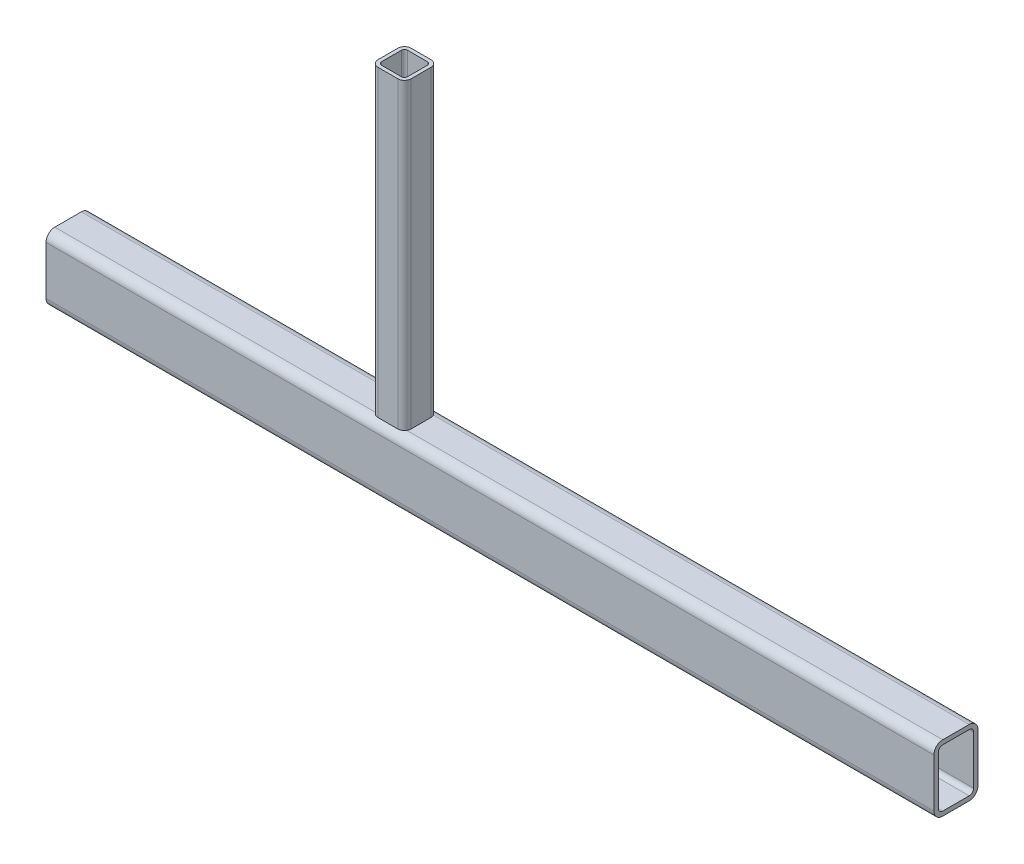
SolidWorks part; units mm, degrees
material "Q235B"
ref_plane "Front Plane" through (0, 0, 0) normal (0, 0, 1) x (1, 0, 0)
ref_plane "Top Plane" through (0, 0, 0) normal (0, 1, 0) x (1, 0, 0)
ref_plane "Right Plane" through (0, 0, 0) normal (1, 0, 0) x (0, 0, -1)
sketch "Sketch1" plane through (0, 0, 0) normal (0, 0, 1) x (1, 0, 0)
  line L0 (0, 0) -> (805, 0)
  line L1 (305, 0) -> (305, 305)
  dimension "D1" = 805
  dimension "D2" = 305
  dimension "D3" = 305
other "GB/T 6728-2002 rectangular hollow section 60X40X4(1)"
ref_plane "Plane1" through (0, 0, 0) normal (1, 0, 0) x (0, 0, 1)
sketch "Sketch12" plane through (0, 0, 0) normal (1, 0, 0) x (0, 0, 1)
  line L0 (-12, -26) -> (12, -26)
  line L1 (-16, -22) -> (-16, 22)
  line L2 (12, 26) -> (-12, 26)
  line L3 (16, 22) -> (16, -22)
  line L4 (-12, -30) -> (12, -30)
  line L5 (-20, -22) -> (-20, 22)
  line L6 (12, 30) -> (-12, 30)
  line L7 (20, 22) -> (20, -22)
  arc A0 (20, 22) -> (12, 30) centre (12, 22) ccw
  arc A1 (12, -30) -> (20, -22) centre (12, -22) ccw
  arc A2 (-20, -22) -> (-12, -30) centre (-12, -22) ccw
  arc A3 (-12, 30) -> (-20, 22) centre (-12, 22) ccw
  arc A4 (-12, 26) -> (-16, 22) centre (-12, 22) ccw
  arc A5 (16, 22) -> (12, 26) centre (12, 22) ccw
  arc A6 (12, -26) -> (16, -22) centre (12, -22) ccw
  arc A7 (-16, -22) -> (-12, -26) centre (-12, -22) ccw
  point P0 (0, 30)
  point P1 (20, 0)
  point P2 (0, -30)
  point P3 (-20, 0)
  point P4 (-20, 30)
  point P5 (20, 30)
  point P6 (20, -30)
  point P7 (-20, -30)
  point P8 (0, 0)
  point P33 (0, 0)
  dimension "D1" = 8
  dimension "Thickness" = 4
  dimension "V_leg" = 60
  dimension "H_leg" = 40
other "GB/T 6728-2002 square hollow section 30×3.2(1)"
ref_plane "Plane3" through (305, 0, 0) normal (0, 1, 0) x (-1, 0, 0)
sketch "Sketch16" plane through (305, 0, 0) normal (0, 1, 0) x (-1, 0, 0)
  line L0 (-9, -11.8) -> (9, -11.8)
  line L1 (-11.8, -9) -> (-11.8, 9)
  line L2 (9, 11.8) -> (-9, 11.8)
  line L3 (11.8, 9) -> (11.8, -9)
  line L4 (-9, -15) -> (9, -15)
  line L5 (-15, -9) -> (-15, 9)
  line L6 (9, 15) -> (-9, 15)
  line L7 (15, 9) -> (15, -9)
  arc A0 (15, 9) -> (9, 15) centre (9, 9) ccw
  arc A1 (9, -15) -> (15, -9) centre (9, -9) ccw
  arc A2 (-15, -9) -> (-9, -15) centre (-9, -9) ccw
  arc A3 (-9, 15) -> (-15, 9) centre (-9, 9) ccw
  arc A4 (-9, 11.8) -> (-11.8, 9) centre (-9, 9) ccw
  arc A5 (11.8, 9) -> (9, 11.8) centre (9, 9) ccw
  arc A6 (9, -11.8) -> (11.8, -9) centre (9, -9) ccw
  arc A7 (-11.8, -9) -> (-9, -11.8) centre (-9, -9) ccw
  point P0 (-15, 0)
  point P1 (15, 0)
  point P2 (0, 15)
  point P3 (0, -15)
  point P4 (0, 0)
  point P5 (-15, -15)
  point P6 (15, -15)
  point P7 (15, 15)
  point P8 (-15, 15)
  point P33 (0, 0)
  dimension "D1" = 6
  dimension "Thickness" = 3.2
  dimension "V_leg" = 30
other "Trim/Extend1"
